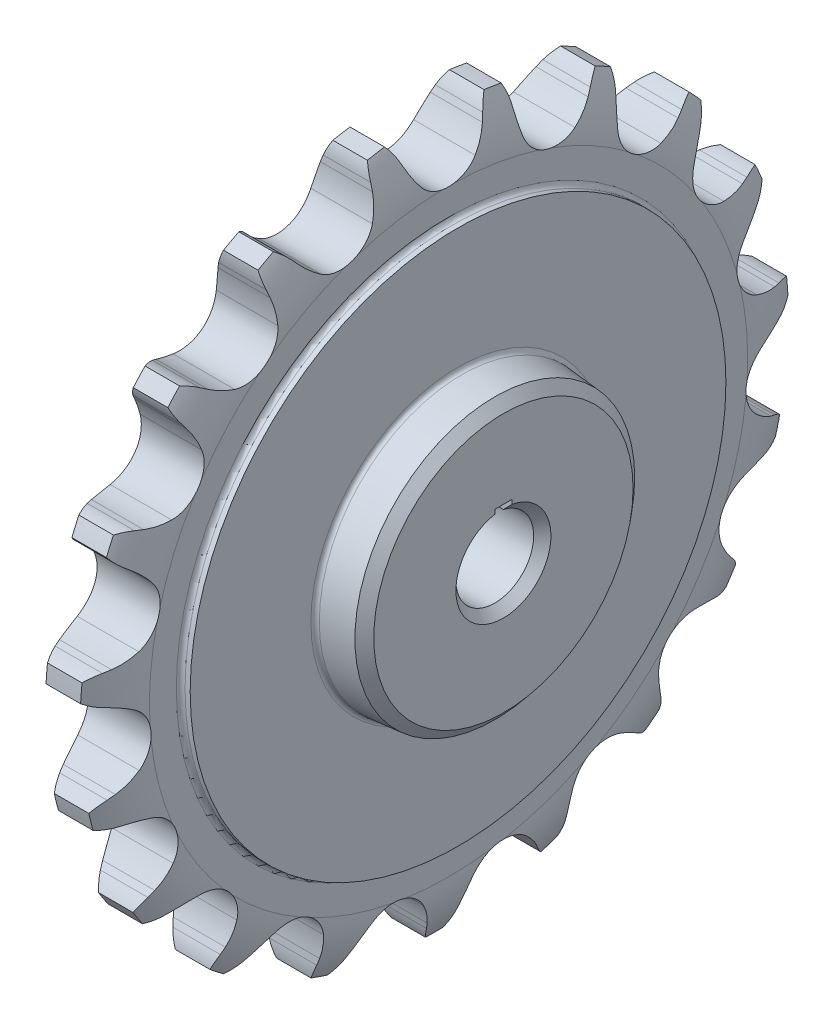
SolidWorks part; units mm, degrees
material "AISI 304"
ref_plane "Front Plane" through (0, 0, 0) normal (0, 0, 1) x (1, 0, 0)
ref_plane "Top Plane" through (0, 0, 0) normal (0, 1, 0) x (1, 0, 0)
ref_plane "Right Plane" through (0, 0, 0) normal (1, 0, 0) x (0, 0, -1)
sketch "Sketch1" plane through (0, 0, 0) normal (0, 0, 1) x (1, 0, 0)
  line L0 (-6.35, 0) -> (6.35, 0) construction
  line L1 (-4.75, 4.5) -> (-4.75, 31)
  line L2 (-4.75, 31) -> (-4.1583, 31)
  line L3 (-3.6503, 31.508) -> (-3.6503, 34.6196)
  line L4 (-1.9993, 41) -> (1.9993, 41)
  line L5 (3.6503, 34.6196) -> (3.6503, 31.508)
  line L6 (4.1583, 31) -> (4.75, 31)
  line L7 (4.75, 31) -> (4.75, 4.5)
  line L8 (4.75, 4.5) -> (-4.75, 4.5)
  line L9 (0, 0) -> (0, 41) construction
  line L10 (-3.0556, 38.5796) -> (3.0556, 38.5796) construction
  line L11 (-3.0556, -38.5796) -> (3.0556, -38.5796) construction
  line L12 (6.35, 0) -> (25.35, 0) construction
  line L13 (-3.6503, 34.6196) -> (3.7984, 34.6196) construction
  line L14 (-3.6503, -34.6196) -> (3.7984, -34.6196) construction
  line L15 (25.35, 0) -> (33.27, 0) construction
  line L16 (33.27, 0) -> (45.34, 0) construction
  line L17 (45.34, 0) -> (53.19, 0) construction
  line L18 (53.19, 0) -> (67.57, 0) construction
  arc A0 (-1.9993, 41) -> (-3.6503, 34.6196) centre (9.0492, 34.7373) ccw
  arc A1 (1.9993, 41) -> (3.6503, 34.6196) centre (-9.0492, 34.7373) cw
  arc A2 (3.6503, 31.508) -> (4.1583, 31) centre (4.1583, 31.508) ccw
  arc A3 (-4.1583, 31) -> (-3.6503, 31.508) centre (-4.1583, 31.508) ccw
  point P30 (3.6503, 31)
  point P33 (-3.6503, 31)
  dimension "rx" = 12.7
  dimension "D3" = 0.508
  dimension "d" = 77.1593
  dimension "p" = 12.7
  dimension "z" = 19
  dimension "da" = 82
  dimension "df" = 69.2393
  dimension "dr" = 7.92
  dimension "dk" = 9
  dimension "dg" = 62
  dimension "h" = 12.07
  dimension "bf1" = 7.3005
  dimension "b1" = 7.85
  dimension "ba" = 1.651
  dimension "pt" = 14.38
  dimension "t" = 9.5
revolve "Revolve1" add sketch "Sketch1" angle 360 about L0
sketch "Sketch2" plane through (0, 0, 0) normal (1, 0, 0) x (0, 0, -1)
  line L0 (0, 0) -> (0, 41) construction
  line L1 (0, 0) -> (-6.7484, 40.4408) construction
  line L2 (0, 0) -> (-13.3127, 38.7785) construction
  line L3 (3.1687, 36.0899) -> (0.6738, 38.0502) construction
  line L4 (4.5522, 38.4265) -> (-4.9821, 42.4942) construction
  line L5 (0, 0) -> (6.7484, 40.4408) construction
  line L6 (4.5522, 38.4265) -> (4.8587, 39.1448)
  line L7 (-4.5522, 38.4265) -> (-4.8587, 39.1448)
  circle A0 centre (0, 0) radius 41 construction
  arc A1 (3.1687, 36.0899) -> (-3.1687, 36.0899) centre (0, 38.5796) cw
  arc A2 (3.1687, 36.0899) -> (4.5522, 38.4265) centre (-4.9821, 42.4942) ccw
  arc A3 (5.7509, 40.5947) -> (4.8587, 39.1448) centre (10.1556, 36.885) ccw
  arc A4 (-3.1687, 36.0899) -> (-4.5522, 38.4265) centre (4.9821, 42.4942) cw
  arc A5 (-5.7509, 40.5947) -> (-4.8587, 39.1448) centre (-10.1556, 36.885) cw
  arc A7 (5.7509, 40.5947) -> (-5.7509, 40.5947) centre (0, 0) ccw
  dimension "r1" = 4.0298
  dimension "r3" = 5.7588
  dimension "D1" = 18.947
  dimension "D2" = 9.474
  dimension "α/2" = 51.842
  dimension "M" = 4.9821
  dimension "T" = 3.9146
  dimension "β" = 15.053
  dimension "γ/2" = 13.632
  dimension "bc" = 0.781
extrude "Cut-Extrude1" cut sketch "Sketch2" against normal mid plane 9.5
pattern_circular "CirPattern1" count 19 over 360 about axis through (0, 0, 0) along (1, 0, 0) of "Cut-Extrude1"
sketch "Sketch4" plane through (-4.75, 0, 0) normal (-1, 0, 0) x (0, 0, 1)
  line L1 (-1, 4.3875) -> (1, 4.3875)
  line L2 (-1, 4.3875) -> (-1, 5.9)
  line L3 (-1, 5.9) -> (1, 5.9)
  line L4 (1, 4.3875) -> (1, 5.9)
  circle A0 centre (0, 0) radius 4.5 construction
  point P6 (0, 5.9)
  dimension "D1" = 10.4
  dimension "键槽宽度" = 2
  dimension "t1" = 1
sketch "Sketch5" plane through (0, 0, 0) normal (0, 0, 1) x (1, 0, 0)
  line L1 (-10, 4.5) -> (10, 4.5)
  line L2 (-10, 4.5) -> (-10, 16.1049)
  line L3 (-10, 16.1049) -> (-4.75, 16.5642)
  line L4 (10, 4.5) -> (10, 16.1049)
  line L6 (0, 0) -> (0, -4.2677) construction
  line L7 (0, 0) -> (-10.4728, 0) construction
  line L8 (-4.75, 4.5) -> (-4.75, 31) construction
  line L9 (-4.75, 16.5642) -> (4.75, 16.5642)
  line L10 (4.75, 31) -> (4.75, 4.5) construction
  line L11 (4.75, 16.5642) -> (10, 16.1049)
  dimension "D1" = 5
  dimension "L" = 20
  dimension "H" = 11.6049
revolve "Revolve2" add sketch "Sketch5" angle 360 about L7
extrude "Cut-Extrude2" cut sketch "Sketch4" against normal through all
mirror "Mirror1" about plane through (0, 0, 0) normal (1, 0, 0) of "Cut-Extrude2"
fillet "Fillet1" radius 0.508 2 edges at (4.75, 0, -16.5642) (-4.75, 0, -16.5642)
chamfer "Chamfer1" distance 1 angle 45 4 edges at (10, -4.5, 0) (10, 0, -16.1049) (-10, -4.5, 0) (-10, 0, -16.1049)
